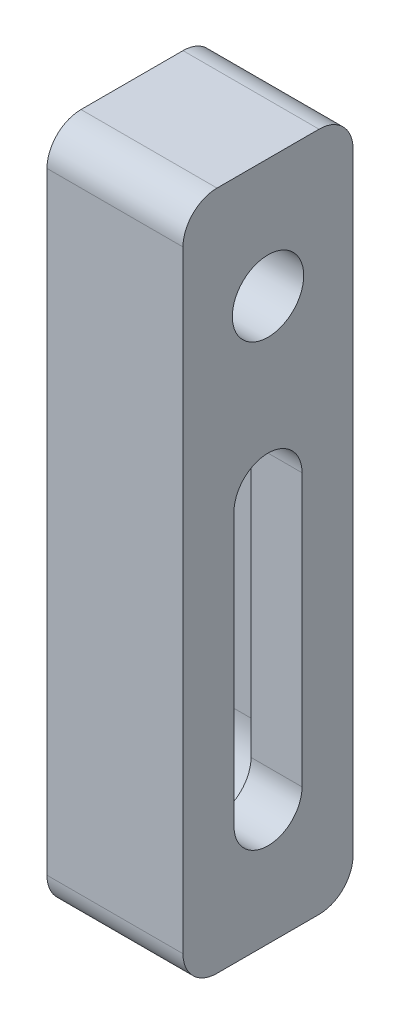
from build123d import *

# Parameters (mm, degrees)
SKETCH_1_W             = 8
SKETCH_1_H             = 40
EXTRUDE_1_DEPTH        = 10
HOLE_WIZARD_M5_1_D     = 4.2
HOLE_WIZARD_M5_1_DEPTH = 12.4
HOLE_WIZARD_M5_1_TIP   = 1.2618073
FILLET_1_R             = 2
CUT_EXTRUDE_1_DEPTH    = 51.185056966
CUT_EXTRUDE_2_DEPTH    = 5
FILLET_2_R             = 2


with BuildPart() as part:
    # 草图1 → 凸台-拉伸1 (new body)
    with BuildSketch(Plane.XY):
        with Locations((-5.75595287, 28.523601913)):
            Rectangle(SKETCH_1_W, SKETCH_1_H)
    extrude(amount=EXTRUDE_1_DEPTH)

    # M5 螺纹孔1
    with Locations(Plane(origin=(-1.75595287, 0, 0), x_dir=(0, 0, -1), z_dir=(1, 0, 0))):
        with Locations((-5, 41.523601913)):
            Hole(HOLE_WIZARD_M5_1_D / 2, depth=HOLE_WIZARD_M5_1_DEPTH)
            with Locations((0, 0, -(HOLE_WIZARD_M5_1_DEPTH + HOLE_WIZARD_M5_1_TIP / 2))):  # 118° drill point
                Cone(0, HOLE_WIZARD_M5_1_D / 2, HOLE_WIZARD_M5_1_TIP, mode=Mode.SUBTRACT)

    # 圆角1
    fillet_1_edges = [part.edges().sort_by_distance(p)[0] for p in [
        (-5.75595287, 48.523601913, 10),
        (-5.75595287, 48.523601913, 0),
    ]]
    fillet(fillet_1_edges, radius=FILLET_1_R)

    # 草图5 → 切除-拉伸1 (cut, through all)
    with BuildSketch(Plane.ZY.offset(9.75595287)):
        with BuildLine():
            Line((3, 15.523601913), (3, 31.523601913))
            ThreePointArc((3, 31.523601913), (5, 33.523601913), (7, 31.523601913))
            Line((7, 31.523601913), (7, 15.523601913))
            ThreePointArc((7, 15.523601913), (5, 13.523601913), (3, 15.523601913))
        make_face()
    extrude(amount=-CUT_EXTRUDE_1_DEPTH, mode=Mode.SUBTRACT)

    # 草图6 → 切除-拉伸2 (cut)
    with BuildSketch(Plane.ZY.offset(9.75595287)):
        with BuildLine():
            Line((9, 31.523601913), (9, 15.523601913))
            ThreePointArc((9, 15.523601913), (5, 11.523601913), (1, 15.523601913))
            Line((1, 15.523601913), (1, 31.523601913))
            ThreePointArc((1, 31.523601913), (5, 35.523601913), (9, 31.523601913))
        make_face()
    extrude(amount=-CUT_EXTRUDE_2_DEPTH, mode=Mode.SUBTRACT)

    # 圆角2
    fillet_2_edges = [part.edges().sort_by_distance(p)[0] for p in [
        (-5.75595287, 8.523601913, 10),
        (-5.75595287, 8.523601913, 0),
    ]]
    fillet(fillet_2_edges, radius=FILLET_2_R)


solid = part.part
